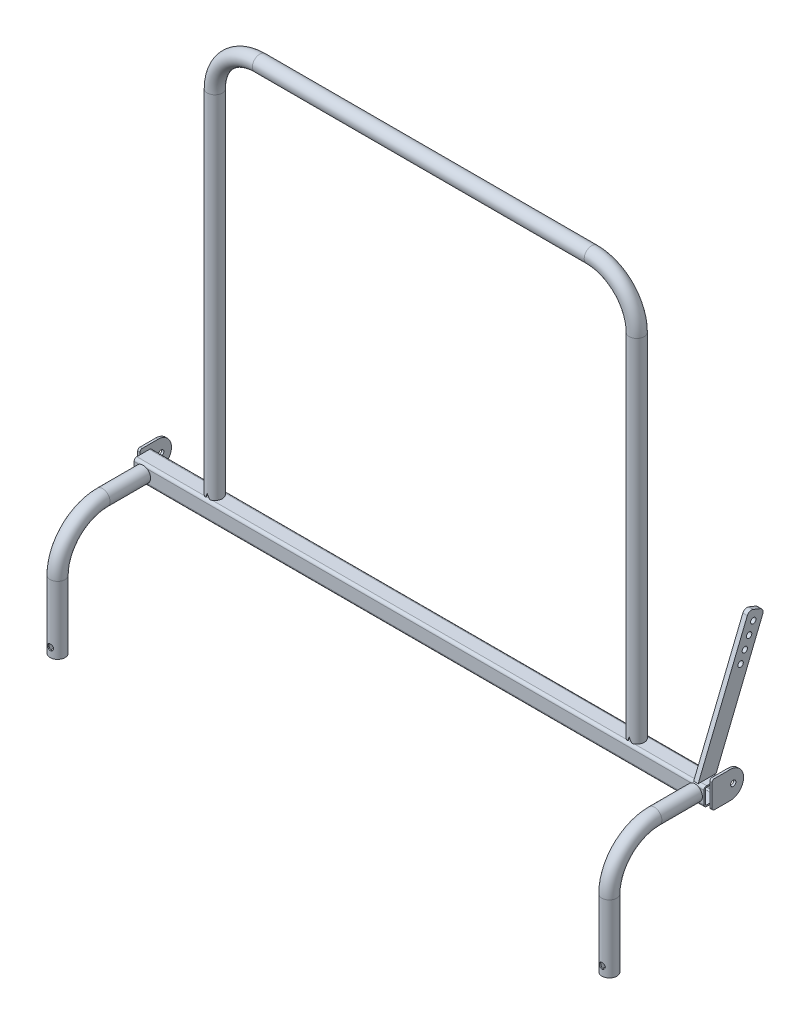
SolidWorks part; units mm, degrees
material "普通碳钢"
ref_plane "前视基准面" through (0, 0, 0) normal (0, 0, 1) x (1, 0, 0)
ref_plane "上视基准面" through (0, 0, 0) normal (0, 1, 0) x (1, 0, 0)
ref_plane "右视基准面" through (0, 0, 0) normal (1, 0, 0) x (0, 0, -1)
sketch3d "3D草图1"
  line L0 (-632.5, 0, 0) -> (632.5, 0, 0)
  line L1 (-473.35, 0, 0) -> (-473.35, 800, 0)
  line L2 (-373.35, 900, 0) -> (363.35, 900, 0)
  line L3 (463.35, 800, 0) -> (463.35, 0, 0)
  line L4 (-612.5, 0, 0) -> (-612.5, 0, 110)
  line L5 (-612.5, -100, 210) -> (-612.5, -250, 210)
  line L6 (612.5, 0, 0) -> (612.5, 0, 110)
  line L7 (612.5, -100, 210) -> (612.5, -250, 210)
  arc A0 (363.35, 900, 0) -> (463.35, 800, 0) centre (363.35, 800, 0) ccw
  arc A1 (-473.35, 800, 0) -> (-373.35, 900, 0) centre (-373.35, 800, 0) ccw
  arc A2 (-612.5, 0, 110) -> (-612.5, -100, 210) centre (-612.5, -100, 110) ccw
  arc A3 (612.5, 0, 110) -> (612.5, -100, 210) centre (612.5, -100, 110) ccw
  point P4 (0, 0, 0)
  point P11 (463.35, 900, 0)
  point P12 (363.35, 800, -100)
  point P15 (-473.35, 900, 0)
  point P16 (-373.35, 800, -100)
  point P22 (-612.5, 0, 210)
  point P23 (-512.5, -100, 110)
  point P29 (612.5, 0, 210)
  point P30 (712.5, -100, 110)
  dimension "D5" = 100
  dimension "D9" = 100
  dimension "D13" = 100
  dimension "D1" = 1265
  dimension "D2" = 900
  dimension "D3" = 936.7
  dimension "D4" = 159.15
  dimension "D6" = 20
  dimension "D7" = 210
  dimension "D8" = 250
  dimension "D10" = 20
  dimension "D11" = 210
  dimension "D12" = 250
other "冷弯空心方管gb∕t6728-2002 40 X 40 X 4(1)"
ref_plane "基准面2" through (-632.5, 0, 0) normal (1, 0, 0) x (0, 0, -1)
sketch "Sketch1" plane through (-632.5, 0, 0) normal (1, 0, 0) x (0, 0, -1)
  line L0 (-14, -17) -> (14, -17)
  line L1 (-17, -14) -> (-17, 14)
  line L2 (14, 17) -> (-14, 17)
  line L3 (17, 14) -> (17, -14)
  line L4 (-14, -20) -> (14, -20)
  line L5 (-20, -14) -> (-20, 14)
  line L6 (14, 20) -> (-14, 20)
  line L7 (20, 14) -> (20, -14)
  arc A0 (20, 14) -> (14, 20) centre (14, 14) ccw
  arc A1 (14, -20) -> (20, -14) centre (14, -14) ccw
  arc A2 (-20, -14) -> (-14, -20) centre (-14, -14) ccw
  arc A3 (-14, 20) -> (-20, 14) centre (-14, 14) ccw
  arc A4 (-14, 17) -> (-17, 14) centre (-14, 14) ccw
  arc A5 (17, 14) -> (14, 17) centre (14, 14) ccw
  arc A6 (14, -17) -> (17, -14) centre (14, -14) ccw
  arc A7 (-17, -14) -> (-14, -17) centre (-14, -14) ccw
  point P0 (-20, 0)
  point P1 (20, 0)
  point P2 (0, 20)
  point P3 (0, -20)
  point P4 (0, 0)
  point P5 (-20, -20)
  point P6 (20, -20)
  point P7 (20, 20)
  point P8 (-20, 20)
  point P33 (0, 0)
  dimension "D1" = 6
  dimension "Thickness" = 3
  dimension "V_leg" = 40
other "冷弯空心圆管gb∕t6728-2002 32 X 2(1)"
ref_plane "基准面3" through (-473.35, 0, 0) normal (0, 1, 0) x (1, 0, 0)
sketch "Sketch11" plane through (-473.35, 0, 0) normal (0, 1, 0) x (1, 0, 0)
  circle A0 centre (0, 0) radius 14.15
  circle A1 centre (0, 0) radius 16.65
  point P3 (0, 0)
  dimension "Out_dia" = 33.3
  dimension "D1" = 2.5
  dimension "D2" = 28.3
other "剪裁/延伸1"
other "剪裁/延伸2"
ref_plane "基准面4" through (619.5, 0, 0) normal (1, 0, 0) x (0, 0, -1)
sketch "草图4" plane through (619.5, 0, 0) normal (1, 0, 0) x (0, 0, -1)
  line L0 (20, 20) -> (-19.8612, 20)
  line L2 (14, 20) -> (-14, 20) construction
  line L3 (-19.8612, 20) -> (89.2674, 288.6837)
  line L4 (110.1388, 291) -> (56.6879, 159.3994) construction
  line L6 (20, 20) -> (123.484, 274.7863)
  line L7 (102.2954, 294.1856) -> (117.9821, 287.8143)
  arc A0 (123.484, 274.7863) -> (117.9821, 287.8143) centre (114.2191, 278.5493) ccw
  arc A1 (89.2674, 288.6837) -> (102.2954, 294.1856) centre (98.5324, 284.9207) cw
  circle A2 centre (102.6127, 272.4701) radius 6
  circle A3 centre (93.205, 249.3077) radius 6
  circle A4 centre (83.7974, 226.1453) radius 6
  circle A5 centre (74.3897, 202.9829) radius 6
  point P17 (127.2471, 284.0512)
  point P20 (93.0305, 297.9487)
  dimension "D3" = 10
  dimension "D4" = 12
  dimension "D1" = 300
  dimension "D2" = 285
  dimension "D5" = 20
  dimension "D6" = 25
  dimension "D7" = 50
  dimension "D8" = 25
extrude "凸台-拉伸1" add sketch "草图4" against normal blind 10 separate body
sketch "草图6" plane through (632.5, 0, 0) normal (1, 0, 0) x (0, 0, -1)
  line L16 (-7, 30) -> (33, 30)
  line L17 (-7, -30) -> (33, -30)
  line L18 (-7, 30) -> (-7, -30)
  line L19 (-17, 14) -> (-17, -14) construction
  line L20 (33, 30) -> (33, -30) construction
  line L21 (20, -14) -> (20, 14) construction
  arc A18 (33, 30) -> (33, -30) centre (33, 0) cw
  circle A19 centre (40, 0) radius 6
  dimension "D6" = 40
  dimension "D3" = 10
  dimension "D4" = 12
  dimension "D1" = 60
  dimension "D2" = 30
  dimension "D5" = 20
extrude "凸台-拉伸3" add sketch "草图6" along normal blind 5 separate body
mirror "镜向1" about plane through (0, 0, 0) normal (1, 0, 0) of bodies 124
ref_plane "基准面5" through (0, 0, 226.65) normal (0, 0, 1) x (1, 0, 0)
sketch "草图8" plane through (0, 0, 226.65) normal (0, 0, 1) x (1, 0, 0)
  line L0 (-629.15, -250) -> (-595.85, -250) construction
  line L1 (0, -192.978) -> (0, 192.978) construction
  line L2 (-629.15, -100) -> (-629.15, -250) construction
  circle A0 centre (-612.4, -230) radius 6.5
  circle A1 centre (612.4, -230) radius 6.5
  dimension "D1" = 13
  dimension "D2" = 20
  dimension "D3" = 16.75
extrude "切除-拉伸1" cut sketch "草图8" against normal blind 35
sketch "草图13" plane through (0, 0, 0) normal (0, 0, 1) x (1, 0, 0)
  line L0 (-490, 20) -> (-456.7, 20) construction
  line L1 (-473.35, 20) -> (-473.35, 30) construction
  line L2 (-473.35, 30) -> (-478.35, 20)
  line L3 (-473.35, 30) -> (-468.35, 20)
  line L4 (-478.35, 20) -> (-468.35, 20)
  line L5 (446.7, 20) -> (480, 20) construction
  line L6 (632.5, 20) -> (-632.5, 20) construction
  line L7 (458.35, 20) -> (468.35, 20)
  line L8 (468.35, 20) -> (463.35, 30)
  line L9 (463.35, 30) -> (458.35, 20)
  line L10 (480, 20) -> (480, 800) construction
  point P16 (463.35, 20)
  dimension "D1" = 10
  dimension "D2" = 10
  dimension "D3" = 5
  dimension "D4" = 10
  dimension "D5" = 10
extrude "切除-拉伸6" cut sketch "草图13" against normal mid plane 80
fillet "圆角1" radius 5 2 edges at (-635, -30, 7) (-635, 30, 7)
fillet "圆角2" radius 5 2 edges at (635, -30, 7) (635, 30, 7)
